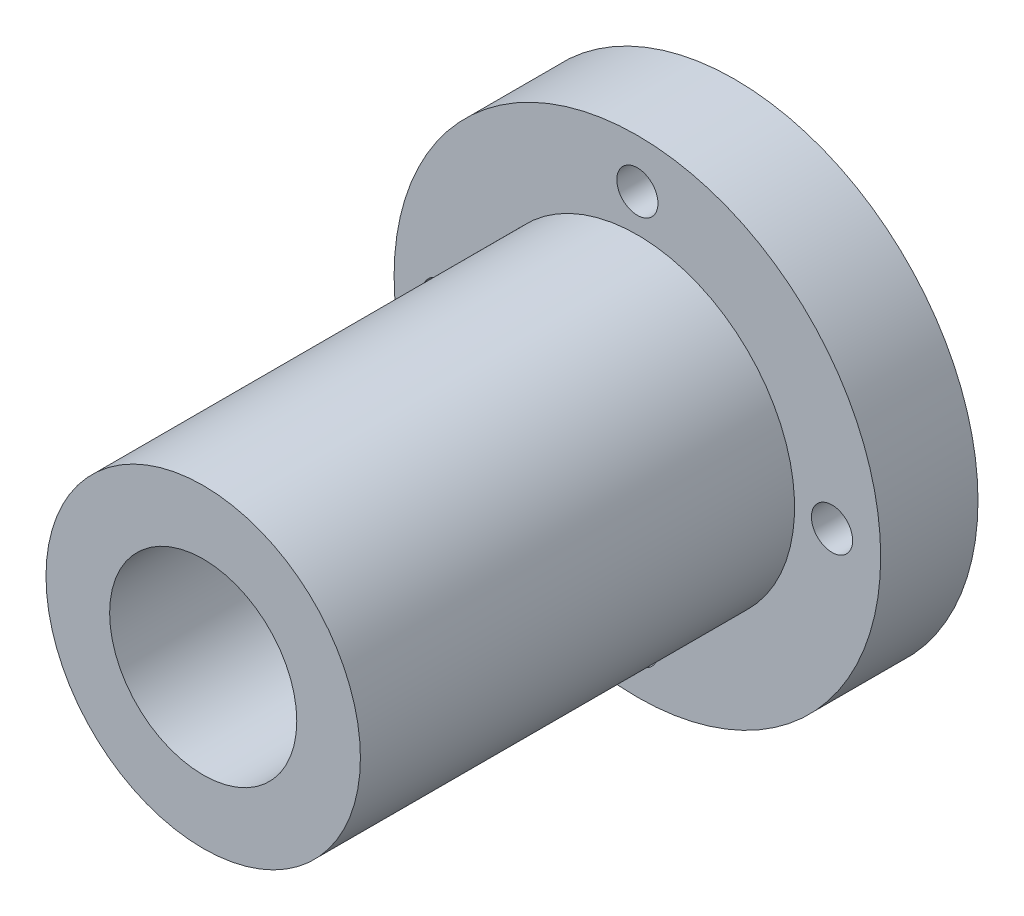
from build123d import *

# Parameters (mm, degrees)
SKETCH_1_R                = 21
SKETCH_1_R_2              = 12.5
EXTRUDE_1_DEPTH           = 71
SKETCH_2_R                = 32.5
SKETCH_2_R_2              = 12.5
EXTRUDE_2_DEPTH           = 13
HOLE_WIZARD_1_D           = 5.5
HOLE_WIZARD_1_CBORE_D     = 10
HOLE_WIZARD_1_CBORE_DEPTH = 5.7


with BuildPart() as part:
    # 草图1 → 凸台-拉伸1 (new body)
    with BuildSketch(Plane.XY):
        Circle(SKETCH_1_R)
        Circle(SKETCH_1_R_2, mode=Mode.SUBTRACT)
    extrude(amount=EXTRUDE_1_DEPTH)

    # 草图2 → 凸台-拉伸2 (add)
    with BuildSketch(Plane(origin=(0, 0, 0), x_dir=(-1, 0, 0), z_dir=(0, 0, -1))):
        Circle(SKETCH_2_R)
        with Locations(Location((0, 0, 0), (0, 0, 180))):
            Circle(SKETCH_2_R_2, mode=Mode.SUBTRACT)
    extrude(amount=-EXTRUDE_2_DEPTH)

    # 打孔尺寸(%根据)内六角圆柱头螺钉的类型1 (through all)
    with Locations(Plane(origin=(0, 26, 0), x_dir=(-1, 0, 0), z_dir=(0, 0, -1))):
        with Locations((0, 0), (26, -26), (0, -52), (-26, -26)):
            CounterBoreHole(HOLE_WIZARD_1_D / 2, HOLE_WIZARD_1_CBORE_D / 2, HOLE_WIZARD_1_CBORE_DEPTH)


solid = part.part
